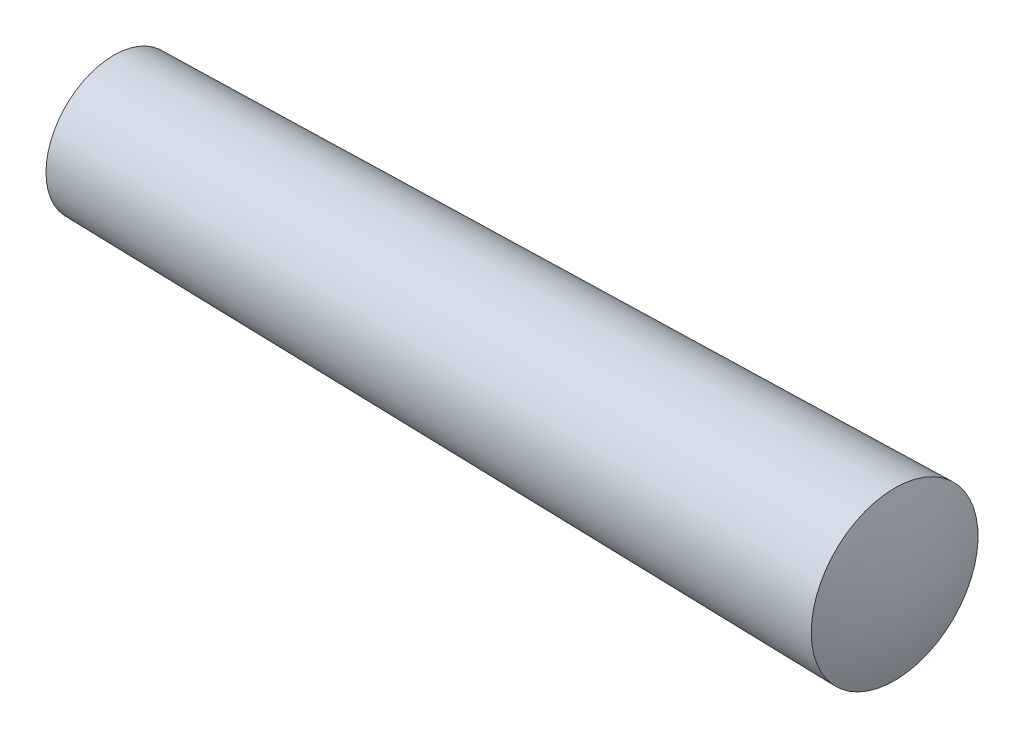
SolidWorks part; units mm, degrees
ref_plane "Front" through (0, 0, 0) normal (0, 0, 1) x (1, 0, 0)
ref_plane "Top" through (0, 0, 0) normal (0, 1, 0) x (1, 0, 0)
ref_plane "Right" through (0, 0, 0) normal (1, 0, 0) x (0, 0, -1)
other "Configuration Table"
sketch "Sketch1" plane through (0, 0, 0) normal (0, 0, 1) x (1, 0, 0)
  line L0 (0, 0) -> (60, 0)
  line L1 (1.2, 5) -> (58.8, 5) construction
  line L2 (58.8, 5) -> (58.8, 6.152) construction
  line L3 (1.2, 5) -> (58.8, 6.152)
  line L4 (-4.0035, 0) -> (8.3584, 0) construction
  line L5 (60, 0) -> (60, 3.9125) construction
  line L6 (0, 0) -> (0, -0.8153) construction
  arc A0 (1.2, 5) -> (0, 0) centre (11.0167, 0) ccw
  arc A1 (60, 0) -> (58.8, 6.152) centre (43.6304, 0) ccw
revolve "Base-Revolve" add sketch "Sketch1" angle 360 about L4
equation "\"D5@Sketch1\" = ( \"l@Sketch1\"-2*\"a@Sketch1\")/ 50"
equation "\"a1@Sketch1\" = \"a@Sketch1\""
